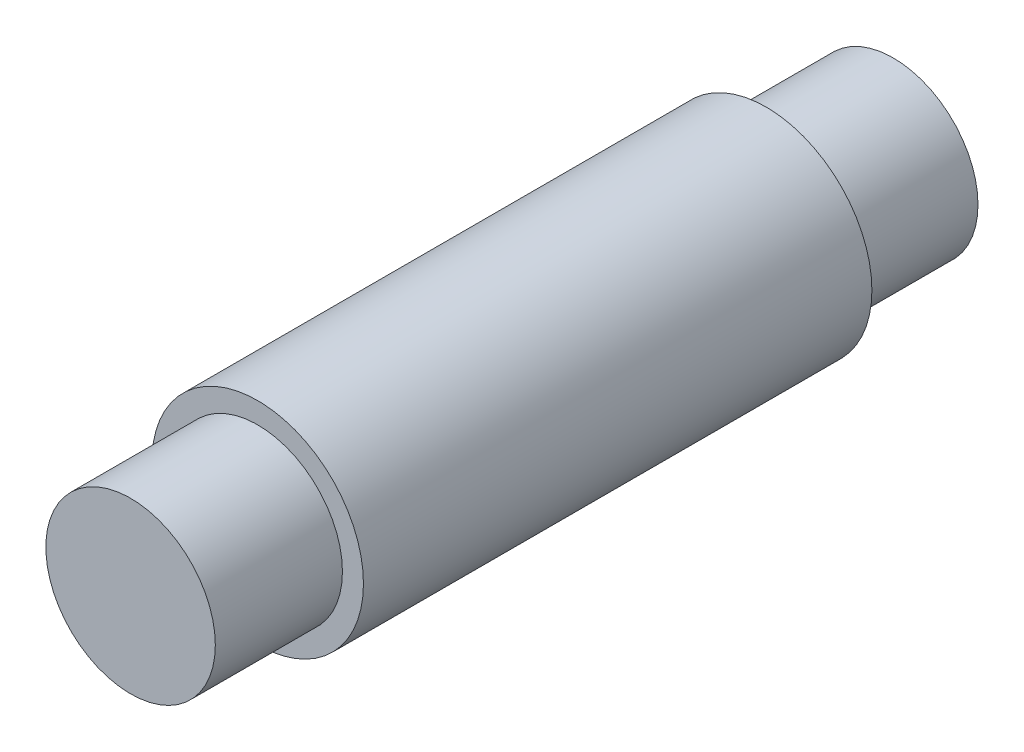
from build123d import *

# Parameters (mm, degrees)
BOSS_EXTRUDE1_DEPTH      = 9.525
BOSS_EXTRUDE1_DEPTH_BACK = 9.525
SKETCH1_R                = 3.9624
BOSS_EXTRUDE2_DEPTH      = 14.2875
BOSS_EXTRUDE2_DEPTH_BACK = 14.2875
BOSS_EXTRUDE2_START      = -9.525
SKETCH2_R                = 3.175


with BuildPart() as part:
    # Sketch1 → Boss-Extrude1 (new, two sides: drawn at the far end of the back side and taken through both)
    with BuildSketch(Plane.XY.offset(-BOSS_EXTRUDE1_DEPTH_BACK)):
        Circle(SKETCH1_R)
    extrude(amount=BOSS_EXTRUDE1_DEPTH + BOSS_EXTRUDE1_DEPTH_BACK)

    # Sketch2 → Boss-Extrude2 (add, two sides: drawn at the far end of the back side and taken through both)
    with BuildSketch(Plane.XY.offset(9.525).offset(BOSS_EXTRUDE2_START - BOSS_EXTRUDE2_DEPTH_BACK)):
        Circle(SKETCH2_R)
    extrude(amount=BOSS_EXTRUDE2_DEPTH + BOSS_EXTRUDE2_DEPTH_BACK)


solid = part.part
